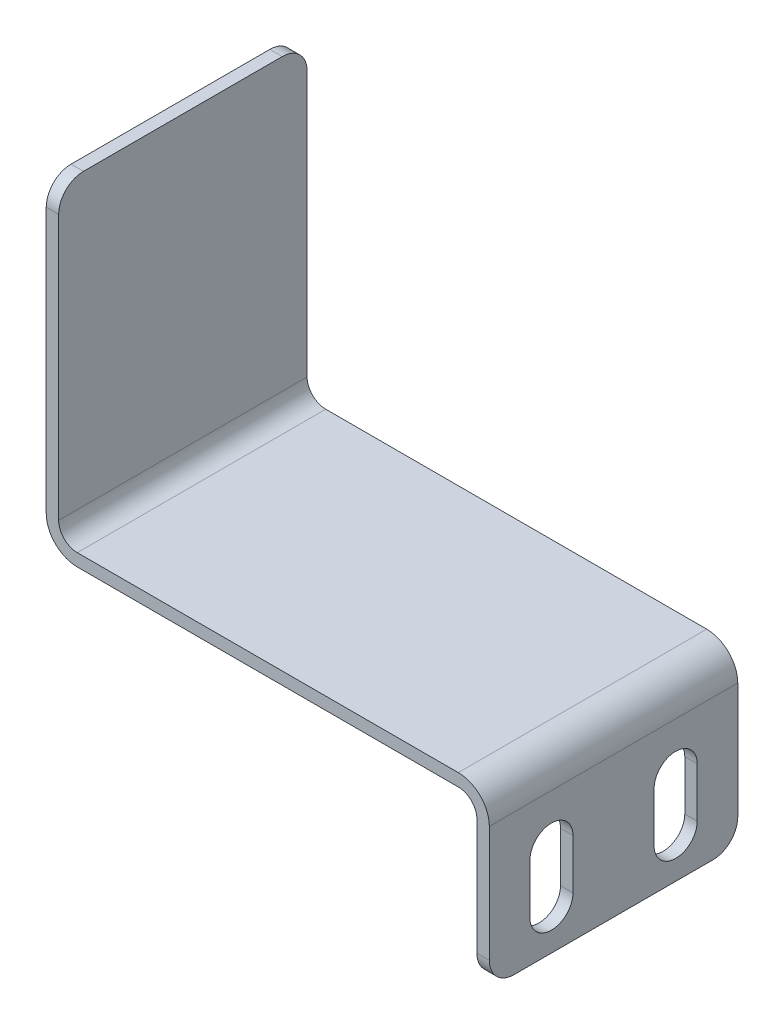
SolidWorks part; units mm, degrees
ref_plane "前视基准面" through (0, 0, 0) normal (0, 0, 1) x (1, 0, 0)
ref_plane "上视基准面" through (0, 0, 0) normal (0, 1, 0) x (1, 0, 0)
ref_plane "右视基准面" through (0, 0, 0) normal (1, 0, 0) x (0, 0, -1)
sketch "草图1" plane through (0, 0, 0) normal (0, 0, 1) x (1, 0, 0)
  line L0 (0, 0) -> (0, 17)
  line L1 (-3, 20) -> (-49, 20)
  line L2 (-52, 23) -> (-52, 58)
  arc A0 (0, 17) -> (-3, 20) centre (-3, 17) ccw
  arc A1 (-49, 20) -> (-52, 23) centre (-49, 23) cw
  point P8 (0, 20)
  point P11 (-52, 20)
  dimension "D5" = 3
  dimension "D1" = 20
  dimension "D2" = 35
  dimension "D4" = 52
extrude "拉伸-薄壁1" add sketch "草图1" along normal blind 30 thin thin type mid plane wall 1.5
fillet "圆角1" radius 3 4 edges at (-52, 58, 0) (-52, 58, 30) (0, 0, 30) (0, 0, 0)
sketch "草图2" plane through (-0.75, 0, 0) normal (-1, 0, 0) x (0, 0, 1)
  line L0 (7.5, 11) -> (7.5, 5) construction
  line L1 (10.1, 11) -> (10.1, 5)
  line L2 (4.9, 11) -> (4.9, 5)
  line L3 (22.5, 11) -> (22.5, 5) construction
  line L4 (25.1, 11) -> (25.1, 5)
  line L5 (19.9, 11) -> (19.9, 5)
  line L6 (15, 0) -> (15, 17.4836) construction
  line L7 (27, 0) -> (3, 0) construction
  arc A0 (10.1, 11) -> (4.9, 11) centre (7.5, 11) ccw
  arc A1 (4.9, 5) -> (10.1, 5) centre (7.5, 5) ccw
  arc A2 (25.1, 11) -> (19.9, 11) centre (22.5, 11) ccw
  arc A3 (19.9, 5) -> (25.1, 5) centre (22.5, 5) ccw
  point P2 (7.5, 8)
  point P7 (22.5, 8)
  dimension "D1" = 15
  dimension "D2" = 5.2
  dimension "D3" = 6
  dimension "D4" = 8
extrude "切除-拉伸1" cut sketch "草图2" against normal blind 10
